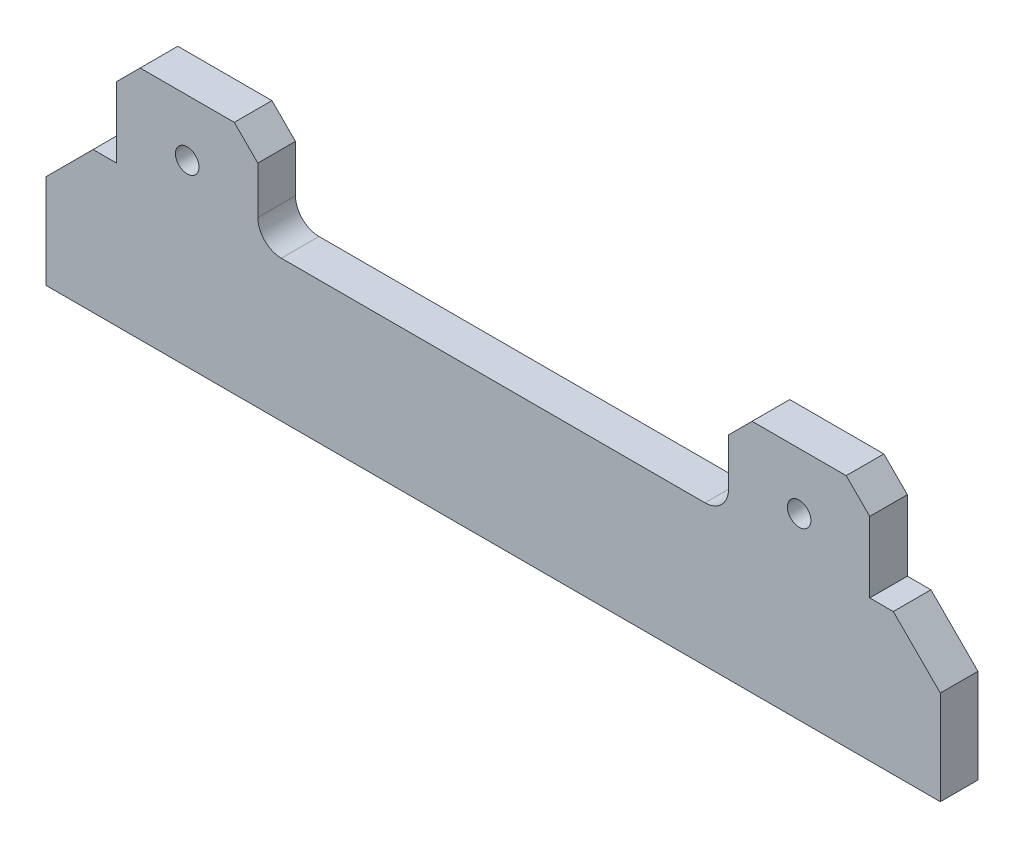
from build123d import *

# Parameters (mm, degrees)
SKETCH_1_W          = 190
SKETCH_1_H          = 50
EXTRUDE_1_DEPTH     = 8
CUT_EXTRUDE_1_DEPTH = 8
CHAMFER_1_SIZE      = 5
HOLE_WIZARD_M6_1_D  = 5
FILLET_1_R          = 5


with BuildPart() as part:
    # 草图1 → 凸台-拉伸1 (new body)
    with BuildSketch(Plane.XY):
        Rectangle(SKETCH_1_W, SKETCH_1_H)
    extrude(amount=EXTRUDE_1_DEPTH)

    # 草图2 → 切除-拉伸1 (cut)
    with BuildSketch(Plane.XY.offset(8)):
        Polygon((-95, -5), (-85, 5), (-80, 5), (-80, 25), (-50, 25), (-50, 5), (50, 5), (50, 25), (80, 25), (80, 5), (85, 5), (95, -5), (95, 25), (-3.801071979, 36.264806318), (-95, 25), align=None)
    extrude(amount=-CUT_EXTRUDE_1_DEPTH, mode=Mode.SUBTRACT)

    # 倒角1
    chamfer_1_edges = [part.edges().sort_by_distance(p)[0] for p in [
        (80, 25, 4),
        (50, 25, 4),
        (-50, 25, 4),
        (-80, 25, 4),
    ]]
    chamfer(chamfer_1_edges, length=CHAMFER_1_SIZE)

    # M6 螺纹孔1 (through all)
    with Locations(Plane.XY.offset(8)):
        with Locations((-65, 13), (65, 13)):
            Hole(HOLE_WIZARD_M6_1_D / 2)

    # 圆角1
    fillet_1_edges = [part.edges().sort_by_distance(p)[0] for p in [
        (50, 5, 4),
        (-50, 5, 4),
    ]]
    fillet(fillet_1_edges, radius=FILLET_1_R)


solid = part.part
